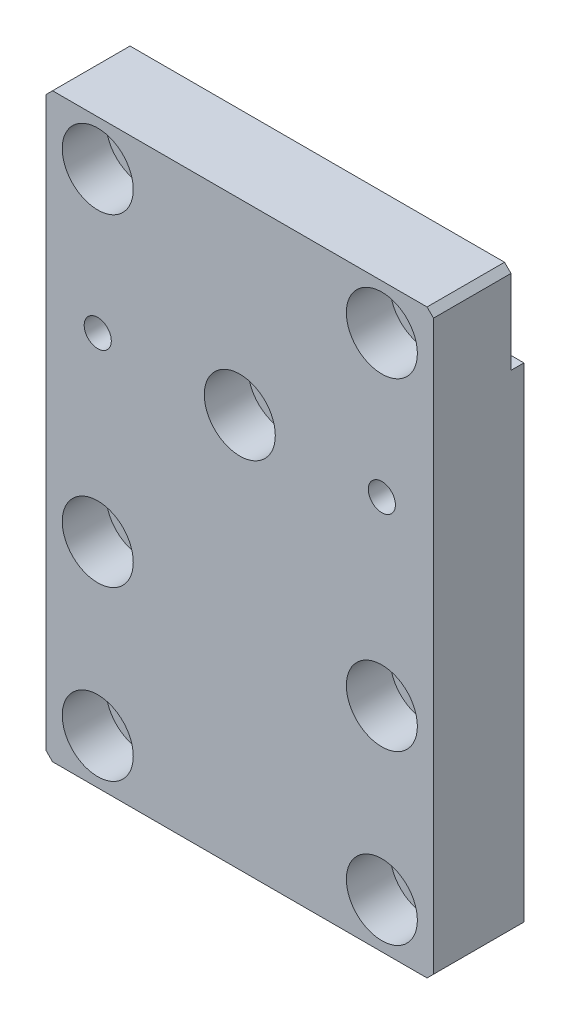
SolidWorks part; units mm, degrees
material "AL6061"
ref_plane "Front Plane" through (0, 0, 0) normal (0, 0, 1) x (1, 0, 0)
ref_plane "Top Plane" through (0, 0, 0) normal (0, 1, 0) x (1, 0, 0)
ref_plane "Right Plane" through (0, 0, 0) normal (1, 0, 0) x (0, 0, -1)
sketch "Sketch1" plane through (0, 0, 0) normal (0, 0, 1) x (1, 0, 0)
  line L1 (-30, -45) -> (30, -45)
  line L2 (-30, -45) -> (-30, 45)
  line L3 (-30, 45) -> (30, 45)
  line L4 (30, -45) -> (30, 45)
  line L5 (-30, -45) -> (30, 45) construction
  line L6 (-30, 45) -> (30, -45) construction
  point P0 (0, 0)
  dimension "D1" = 90
  dimension "D2" = 60
extrude "Boss-Extrude1" add sketch "Sketch1" along normal mid plane 14
sketch "Sketch2" plane through (0, 0, -7) normal (0, 0, -1) x (-1, 0, 0)
  line L0 (30, 45) -> (30, -45) construction
  line L1 (-30, 45) -> (30, 45)
  line L2 (-30, 45) -> (-30, 31)
  line L3 (-30, 31) -> (30, 31)
  line L4 (30, 45) -> (30, 31)
  dimension "D1" = 14
extrude "Cut-Extrude1" cut sketch "Sketch2" against normal blind 2
hole_wizard "Hole Size per Socket Head Cap Screw Type1" positions "Sketch3" profile "Sketch4" counterbore size "M6" standard "GB" end condition through all
sketch "Sketch3" plane through (0, 0, 7) normal (0, 0, 1) x (1, 0, 0)
  line L0 (0, 0) -> (0, 65.8582) construction
  line L3 (-33.7575, 38) -> (45.7693, 38) construction
  line L6 (30, 45) -> (-30, 45) construction
  line L8 (-22, -12) -> (22, -12)
  line L9 (-22, -12) -> (-22, -38)
  line L10 (-22, -38) -> (22, -38)
  line L11 (22, -12) -> (22, -38)
  line L12 (-30, -45) -> (30, -45) construction
  point P13 (-22, 38)
  point P16 (22, 38)
  point P18 (-22, -12)
  point P19 (22, -38)
  point P200 (-22, -38)
  point P201 (22, -12)
  point P214 (0, 16)
  dimension "D1" = 7
  dimension "D2" = 44
  dimension "D3" = 7
  dimension "D4" = 26
  dimension "D5" = 29
sketch "Sketch4" plane through (0, 16, 7) normal (1, 0, 0) x (0, -1, 0)
  line L0 (0, 0) -> (0, 14)
  line L1 (0, 14) -> (3.3, 14)
  line L3 (3.3, 14) -> (3.3, 6.8)
  line L4 (3.3, 6.8) -> (5.5, 6.8)
  line L5 (5.5, 6.8) -> (5.5, 0)
  line L7 (5.5, 0) -> (0, 0)
  line L11 (0, -6.35) -> (0, 107.95) construction
  dimension "通孔孔直径" = 6.6
  dimension "通孔孔深度" = 14
  dimension "柱形沉头孔直径" = 11
  dimension "柱形沉头孔深度" = 6.8
chamfer "Chamfer1" distance 1 angle 45 4 edges at (30, -45, 0) (-30, -45, 0) (30, 45, 1) (-30, 45, 1)
hole_wizard "M5 Tapped Hole1" positions "Sketch5" profile "Sketch6" tap size "M5" standard "GB" end condition through all
sketch "Sketch5" plane through (0, 0, 7) normal (0, 0, 1) x (1, 0, 0)
  line L0 (0, 0) -> (0, 61.5433) construction
  line L1 (-22, 38) -> (-22, -12) construction
  line L4 (29, 45) -> (-29, 45) construction
  point P7 (-22, 16)
  point P10 (22, 16)
  dimension "D1" = 29
sketch "Sketch6" plane through (22, 16, 7) normal (1, 0, 0) x (0, -1, 0)
  line L0 (0, 0) -> (0, 14)
  line L1 (0, 14) -> (2.1, 14)
  line L2 (2.1, 14) -> (2.1, 0)
  line L5 (2.1, 0) -> (0, 0)
  line L11 (0, -6.35) -> (0, 107.95) construction
  dimension "通孔螺纹孔钻头直径" = 4.2
  dimension "通孔螺纹孔钻头深度" = 14
cosmetic thread "Cosmetic Thread1" parameters "D2"=5
cosmetic thread "Cosmetic Thread2" parameters "D2"=5
